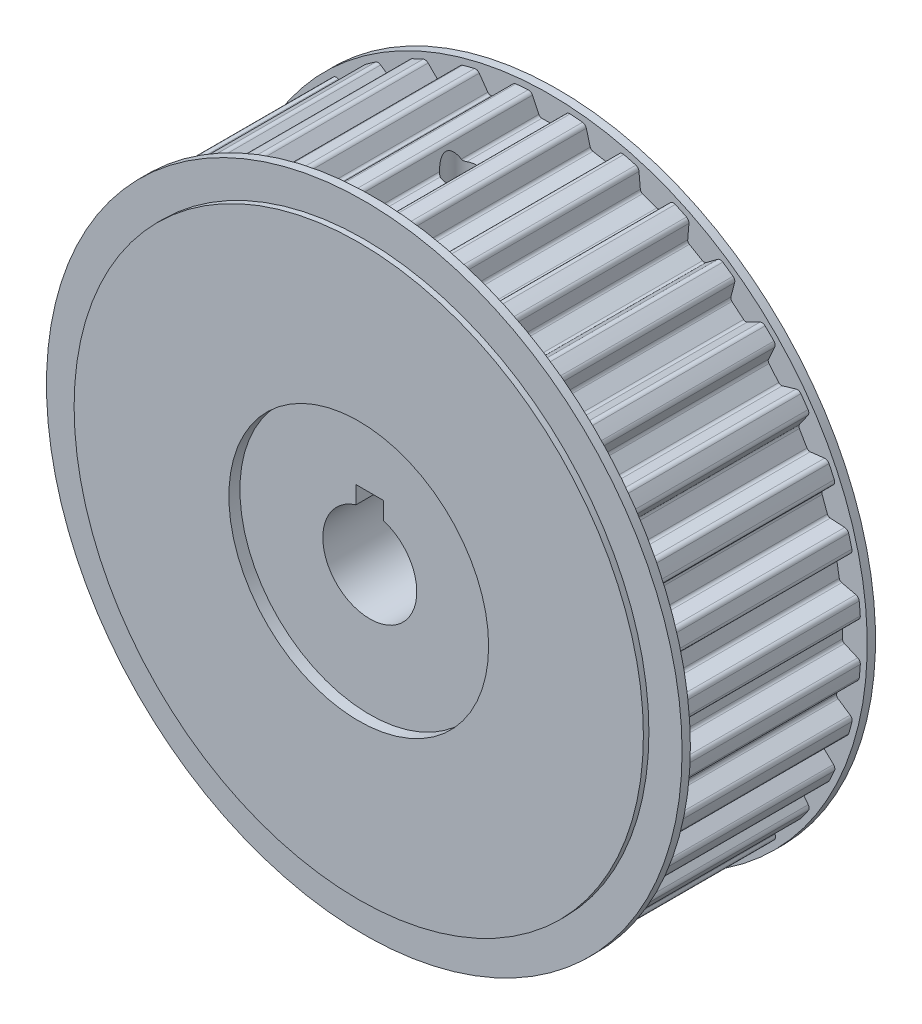
from build123d import *

# Parameters (mm, degrees)
SKETCH_1_R                  = 56.37
EXTRUDE_1_DEPTH             = 18.5
CUT_EXTRUDE_1_DEPTH         = 18.5
PATTERN_CIRCULAR_1_COUNT    = 36
SKETCH_3_R                  = 57.5
EXTRUDE_2_DEPTH             = 2.5
SKETCH_4_R                  = 8.5
CUT_EXTRUDE_2_DEPTH         = 90.339241098
SKETCH_13_OUTSIDE_W         = 150.358
SKETCH_13_OUTSIDE_H         = 150.358
SKETCH_13_OUTSIDE_R         = 51.5
CUT_EXTRUDE_8_DEPTH         = 1
HOLE_WIZARD_M4_1_REACH      = 130.783
HOLE_WIZARD_M4_1_BORE_R     = 1.65
SKETCH_20_W                 = 5
SKETCH_20_H                 = 5.461984524
CUT_EXTRUDE_11_DEPTH        = 90.33924114
SKETCH_21_R                 = 23.5
CUT_EXTRUDE_12_DEPTH        = 2
HOLE_WIZARD_5_5_5_5_2_D     = 5.5
HOLE_WIZARD_5_5_5_5_2_DEPTH = 35
HOLE_WIZARD_5_5_5_5_2_TIP   = 1.652366702


with BuildPart() as part:
    # 草图1 → 凸台-拉伸1 (new, symmetric)
    with BuildSketch(Plane.XY):
        Circle(SKETCH_1_R)
    extrude(amount=EXTRUDE_1_DEPTH, both=True)

    # 草图2 → 切除-拉伸1 (cut, symmetric)
    with BuildSketch(Plane.XY):
        with BuildLine():
            Line((-1.915179338, 53.35175844), (-3.058717591, 55.781753722))
            ThreePointArc((-3.058717591, 55.781753722), (-3.377168746, 56.130786349), (-3.837026152, 56.23925791))
            ThreePointArc((-3.837026152, 56.23925791), (-0.044362039, 56.369982544), (3.748503131, 56.245227569))
            ThreePointArc((3.748503131, 56.245227569), (3.278743817, 56.129989645), (2.961259325, 55.765082548))
            Line((2.961259325, 55.765082548), (1.922823008, 53.368675523))
            ThreePointArc((1.922823008, 53.368675523), (1.701577775, 53.10567219), (1.372289069, 53.007238685))
            Line((1.372289069, 53.007238685), (-1.372289069, 53.007238685))
            ThreePointArc((-1.372289069, 53.007238685), (-1.693779235, 53.100638178), (-1.915179338, 53.35175844))
        make_face()
    cut_extrude_1 = extrude(amount=CUT_EXTRUDE_1_DEPTH, both=True, mode=Mode.SUBTRACT)

    # 阵列(圆周)1: 切除-拉伸1 ×36 about axis
    pattern_circular_1_axis = Axis((0, 0, 0), (0, 0, 1))
    for i in range(1, PATTERN_CIRCULAR_1_COUNT):
        add(cut_extrude_1.rotate(pattern_circular_1_axis, i * 360 / PATTERN_CIRCULAR_1_COUNT), mode=Mode.SUBTRACT)

    # 草图3 → 凸台-拉伸2 (add)
    with BuildSketch(Plane(origin=(0, 0, -18.5), x_dir=(-1, 0, 0), z_dir=(0, 0, -1))):
        Circle(SKETCH_3_R)
    extrude_2 = extrude(amount=-EXTRUDE_2_DEPTH)

    # 镜向1: 凸台-拉伸2 across plane
    add(extrude_2.mirror(Plane.XY))

    # 草图4 → 切除-拉伸2 (cut, through all)
    with BuildSketch(Plane(origin=(0, 0, -18.5), x_dir=(-1, 0, 0), z_dir=(0, 0, -1))):
        Circle(SKETCH_4_R)
    extrude(amount=-CUT_EXTRUDE_2_DEPTH, mode=Mode.SUBTRACT)

    # 草图13 outside → 切除-拉伸8 (cut)
    with BuildSketch(Plane.XY.offset(18.5)):
        Rectangle(SKETCH_13_OUTSIDE_W, SKETCH_13_OUTSIDE_H)
        Circle(SKETCH_13_OUTSIDE_R, mode=Mode.SUBTRACT)
    cut_extrude_8 = extrude(amount=-CUT_EXTRUDE_8_DEPTH, mode=Mode.SUBTRACT)

    # 镜向2: 切除-拉伸8 across plane
    add(cut_extrude_8.mirror(Plane.XY), mode=Mode.SUBTRACT)

    # M4 螺纹孔1 bore → M4 螺纹孔1 (cut, up to next)
    with BuildSketch(Plane(origin=(0, 56.23925791, 0), x_dir=(1, 0, 0), z_dir=(0, 1, 0)), mode=Mode.PRIVATE) as hole_wizard_m4_1_sk1:
        Circle(HOLE_WIZARD_M4_1_BORE_R)
    hole_wizard_m4_1_tool1 = extrude(hole_wizard_m4_1_sk1.sketch, amount=-HOLE_WIZARD_M4_1_REACH, mode=Mode.PRIVATE) & part.part
    add(hole_wizard_m4_1_tool1.solids().sort_by_distance((0, 56.239258, 0))[0], mode=Mode.SUBTRACT)

    # 草图20 → 切除-拉伸11 (cut, through all)
    with BuildSketch(Plane.XY.offset(18.5)):
        with Locations((0, 8.569007738)):
            Rectangle(SKETCH_20_W, SKETCH_20_H)
    extrude(amount=-CUT_EXTRUDE_11_DEPTH, mode=Mode.SUBTRACT)

    # 草图21 → 切除-拉伸12 (cut)
    with BuildSketch(Plane.XY.offset(18.5)):
        Circle(SKETCH_21_R)
    cut_extrude_12 = extrude(amount=-CUT_EXTRUDE_12_DEPTH, mode=Mode.SUBTRACT)

    # 镜向4: 切除-拉伸12 across plane
    add(cut_extrude_12.mirror(Plane.XY), mode=Mode.SUBTRACT)

    # Ø5.5 (5.5) 直径孔2
    with Locations(Plane(origin=(0, 56.23925791, 0), x_dir=(1, 0, 0), z_dir=(0, 1, 0))):
        with Locations((0, 0)):
            Hole(HOLE_WIZARD_5_5_5_5_2_D / 2, depth=HOLE_WIZARD_5_5_5_5_2_DEPTH)
            with Locations((0, 0, -(HOLE_WIZARD_5_5_5_5_2_DEPTH + HOLE_WIZARD_5_5_5_5_2_TIP / 2))):  # 118° drill point
                Cone(0, HOLE_WIZARD_5_5_5_5_2_D / 2, HOLE_WIZARD_5_5_5_5_2_TIP, mode=Mode.SUBTRACT)


solid = part.part
